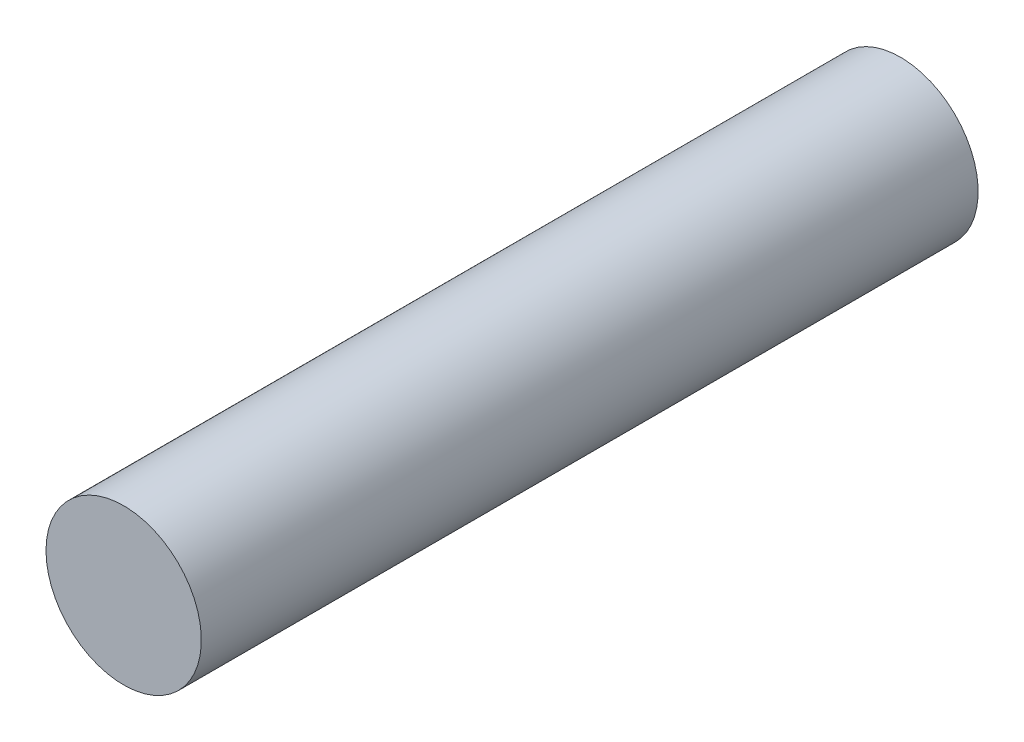
SolidWorks part; units mm, degrees
ref_plane "Front Plane" through (0, 0, 0) normal (0, 0, 1) x (1, 0, 0)
ref_plane "Top Plane" through (0, 0, 0) normal (0, 1, 0) x (1, 0, 0)
ref_plane "Right Plane" through (0, 0, 0) normal (1, 0, 0) x (0, 0, -1)
other "Configuration Table"
ref_plane "Plane1" through (0, 0, 0) normal (0, -1, 0) x (1, 0, 0)
sketch "Sketch1" plane through (0, 0, 0) normal (0, -1, 0) x (1, 0, 0)
  line L0 (7.5, 75) -> (0, 75)
  line L1 (0, 75) -> (0, 0)
  line L2 (0, 0) -> (7.5, 0)
  line L3 (7.5, 0) -> (7.5, 75)
  line L4 (0, 75) -> (0, 0) construction
revolve "Revolve1" add sketch "Sketch1" angle 360 about L4
